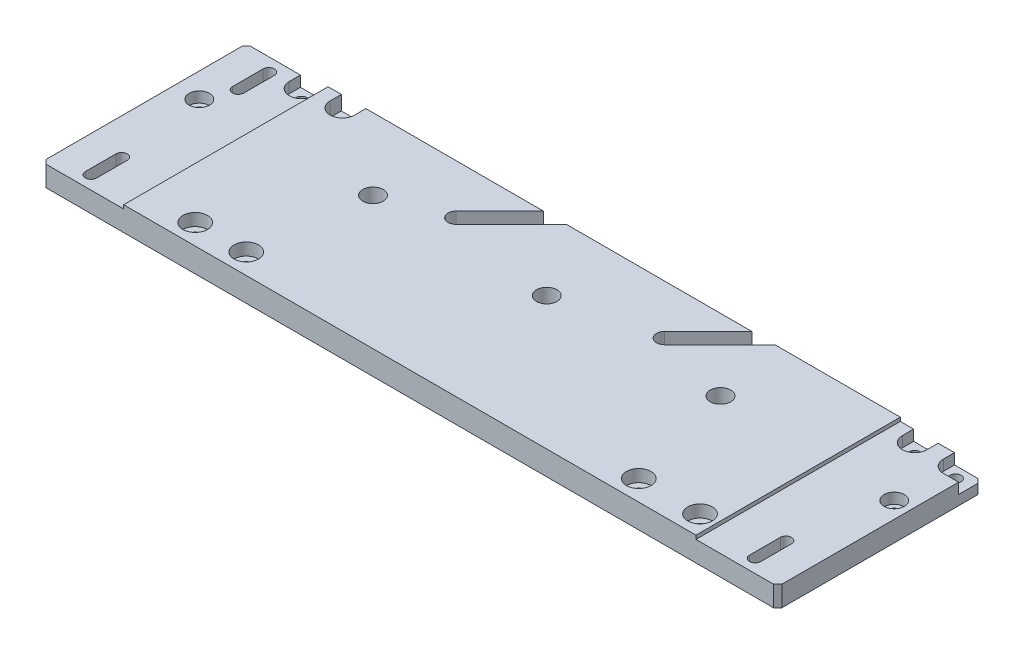
from build123d import *

# Parameters (mm, degrees)
SKETCH1_W           = 360
SKETCH1_H           = 100
BOSS_EXTRUDE1_DEPTH = 10
SKETCH2_W           = 280
SKETCH2_H           = 100
BOSS_EXTRUDE2_DEPTH = 1.8
SKETCH3_R           = 4
CUT_EXTRUDE1_DEPTH  = 188.187713272
CUT_EXTRUDE2_DEPTH  = 39
CUT_EXTRUDE3_DEPTH  = 39
CHAMFER1_SIZE       = 2
SKETCH6_R           = 2.75
CUT_EXTRUDE4_DEPTH  = 188.187713272
SKETCH7_R           = 6
CUT_EXTRUDE5_DEPTH  = 6
SKETCH8_R           = 2.75
CUT_EXTRUDE6_DEPTH  = 19
SKETCH9_R           = 6
CUT_EXTRUDE7_DEPTH  = 7
SKETCH11_W          = 12
SKETCH11_H          = 11.502298529
SKETCH11_H_2        = 11
CUT_EXTRUDE8_DEPTH  = 7
SKETCH12_R          = 2.75
CUT_EXTRUDE9_DEPTH  = 188.187713272
LPATTERN1_COUNT     = 5
LPATTERN1_PITCH     = 85
SKETCH13_R          = 5
CUT_EXTRUDE10_DEPTH = 7
SKETCH14_R          = 2.75
CUT_EXTRUDE11_DEPTH = 10
SKETCH15_R          = 6
CUT_EXTRUDE12_DEPTH = 5.2
SKETCH16_W          = 12
SKETCH16_H          = 11
CUT_EXTRUDE13_DEPTH = 5.2
SKETCH17_W          = 12
SKETCH17_H          = 12
CUT_EXTRUDE14_DEPTH = 5.2


with BuildPart() as part:
    # Sketch1 → Boss-Extrude1 (new body)
    with BuildSketch(Plane(origin=(0, 0, 0), x_dir=(1, 0, 0), z_dir=(0, 1, 0))):
        Rectangle(SKETCH1_W, SKETCH1_H)
    extrude(amount=BOSS_EXTRUDE1_DEPTH)

    # Sketch2 → Boss-Extrude2 (add)
    with BuildSketch(Plane(origin=(0, 10, 0), x_dir=(1, 0, 0), z_dir=(0, 1, 0))):
        Rectangle(SKETCH2_W, SKETCH2_H)
    extrude(amount=BOSS_EXTRUDE2_DEPTH)

    # Sketch3 → Cut-Extrude1 (cut, through all)
    with BuildSketch(Plane.XZ):
        with Locations(Location((-39, -40, 0), (0, 0, 270))):
            Circle(SKETCH3_R)
        with Locations(Location((63, -40, 0), (0, 0, 270))):
            Circle(SKETCH3_R)
    extrude(amount=-CUT_EXTRUDE1_DEPTH, mode=Mode.SUBTRACT)

    # Sketch4 → Cut-Extrude2 (cut)
    with BuildSketch(Plane.XZ):
        with BuildLine():
            Line((51.686291501, -23.029437252), (79.970562748, -51.313708499))
            ThreePointArc((79.970562748, -51.313708499), (79.970562748, -56.970562748), (74.313708499, -56.970562748))
            Line((74.313708499, -56.970562748), (46.029437252, -28.686291501))
            ThreePointArc((46.029437252, -28.686291501), (46.029437252, -23.029437252), (51.686291501, -23.029437252))
        make_face()
        with BuildLine():
            Line((-50.313708499, -23.029437252), (-22.029437252, -51.313708499))
            ThreePointArc((-22.029437252, -51.313708499), (-22.029437252, -56.970562748), (-27.686291501, -56.970562748))
            Line((-27.686291501, -56.970562748), (-55.970562748, -28.686291501))
            ThreePointArc((-55.970562748, -28.686291501), (-55.970562748, -23.029437252), (-50.313708499, -23.029437252))
        make_face()
    extrude(amount=-CUT_EXTRUDE2_DEPTH, mode=Mode.SUBTRACT)

    # Sketch5 → Cut-Extrude3 (cut)
    with BuildSketch(Plane.XZ):
        with BuildLine():
            Line((-159.753978998, 43.501457769), (-159.746021776, 28.501459879))
            ThreePointArc((-159.746021776, 28.501459879), (-162.494562565, 25.750001442), (-165.246021002, 28.498542231))
            Line((-165.246021002, 28.498542231), (-165.253978224, 43.498540121))
            ThreePointArc((-165.253978224, 43.498540121), (-162.505437435, 46.249998558), (-159.753978998, 43.501457769))
        make_face()
        with BuildLine():
            Line((159.75, 43.5), (159.75, 28.5))
            ThreePointArc((159.75, 28.5), (162.5, 25.75), (165.25, 28.5))
            Line((165.25, 28.5), (165.25, 43.5))
            ThreePointArc((165.25, 43.5), (162.5, 46.25), (159.75, 43.5))
        make_face()
        with BuildLine():
            Line((-159.753978998, -43.501457769), (-159.746021776, -28.501459879))
            ThreePointArc((-159.746021776, -28.501459879), (-162.494562565, -25.750001442), (-165.246021002, -28.498542231))
            Line((-165.246021002, -28.498542231), (-165.253978224, -43.498540121))
            ThreePointArc((-165.253978224, -43.498540121), (-162.505437435, -46.249998558), (-159.753978998, -43.501457769))
        make_face()
    extrude(amount=-CUT_EXTRUDE3_DEPTH, mode=Mode.SUBTRACT)

    # Chamfer1
    chamfer1_edges = [part.edges().sort_by_distance(p)[0] for p in [
        (180, 5, 50),
        (-180, 5, 50),
        (-180, 5, -50),
        (180, 5, -50),
    ]]
    chamfer(chamfer1_edges, length=CHAMFER1_SIZE)

    # Sketch6 → Cut-Extrude4 (cut, through all)
    with BuildSketch(Plane(origin=(0, 11.8, 0), x_dir=(1, 0, 0), z_dir=(0, 1, 0))):
        with Locations(Location((132, -40, 0), (0, 0, 270))):
            Circle(SKETCH6_R)
        with Locations(Location((102, -40, 0), (0, 0, 270))):
            Circle(SKETCH6_R)
        with Locations(Location((-90, -40, 0), (0, 0, 270))):
            Circle(SKETCH6_R)
        with Locations(Location((-115, -40, 0), (0, 0, 270))):
            Circle(SKETCH6_R)
    extrude(amount=-CUT_EXTRUDE4_DEPTH, mode=Mode.SUBTRACT)

    # Sketch7 → Cut-Extrude5 (cut)
    with BuildSketch(Plane(origin=(0, 11.8, 0), x_dir=(1, 0, 0), z_dir=(0, 1, 0))):
        with Locations(Location((-115, -40, 0), (0, 0, 270))):
            Circle(SKETCH7_R)
        with Locations(Location((-90, -40, 0), (0, 0, 270))):
            Circle(SKETCH7_R)
        with Locations(Location((102, -40, 0), (0, 0, 270))):
            Circle(SKETCH7_R)
        with Locations(Location((132, -40, 0), (0, 0, 270))):
            Circle(SKETCH7_R)
    extrude(amount=-CUT_EXTRUDE5_DEPTH, mode=Mode.SUBTRACT)

    # Sketch8 → Cut-Extrude6 (cut)
    with BuildSketch(Plane(origin=(0, 11.8, 0), x_dir=(1, 0, 0), z_dir=(0, 1, 0))):
        with Locations(Location((-147.5, 44.5, 0), (0, 0, 270))):
            Circle(SKETCH8_R)
        with Locations(Location((-127.5, 44.5, 0), (0, 0, 270))):
            Circle(SKETCH8_R)
    extrude(amount=-CUT_EXTRUDE6_DEPTH, mode=Mode.SUBTRACT)

    # Sketch9 → Cut-Extrude7 (cut)
    with BuildSketch(Plane(origin=(0, 11.8, 0), x_dir=(1, 0, 0), z_dir=(0, 1, 0))):
        with Locations((-147.5, 44.5)):
            Circle(SKETCH9_R)
        with Locations((-127.5, 44.5)):
            Circle(SKETCH9_R)
    extrude(amount=-CUT_EXTRUDE7_DEPTH, mode=Mode.SUBTRACT)

    # Sketch11 → Cut-Extrude8 (cut)
    with BuildSketch(Plane(origin=(0, 11.8, 0), x_dir=(1, 0, 0), z_dir=(0, 1, 0))):
        with Locations((-147.5, 50.251149265)):
            Rectangle(SKETCH11_W, SKETCH11_H)
        with Locations((-127.5, 50)):
            Rectangle(SKETCH11_W, SKETCH11_H_2)
    extrude(amount=-CUT_EXTRUDE8_DEPTH, mode=Mode.SUBTRACT)

    # Sketch12 → Cut-Extrude9 (cut, through all)
    with BuildSketch(Plane(origin=(0, 11.8, 0), x_dir=(1, 0, 0), z_dir=(0, 1, 0))):
        with Locations(Location((-168, 15, 0), (0, 0, 270))):
            Circle(SKETCH12_R)
    cut_extrude9 = extrude(amount=-CUT_EXTRUDE9_DEPTH, mode=Mode.SUBTRACT)

    # LPattern1: Cut-Extrude9 ×5
    with Locations(*[(i * LPATTERN1_PITCH, 0, 0) for i in range(1, LPATTERN1_COUNT)]):
        add(cut_extrude9, mode=Mode.SUBTRACT)

    # Sketch13 → Cut-Extrude10 (cut)
    with BuildSketch(Plane(origin=(0, 11.8, 0), x_dir=(1, 0, 0), z_dir=(0, 1, 0))):
        with Locations(Location((172, 15, 0), (0, 0, 270))):
            Circle(SKETCH13_R)
        with Locations(Location((87, 15, 0), (0, 0, 270))):
            Circle(SKETCH13_R)
        with Locations(Location((2, 15, 0), (0, 0, 270))):
            Circle(SKETCH13_R)
        with Locations(Location((-83, 15, 0), (0, 0, 270))):
            Circle(SKETCH13_R)
        with Locations(Location((-168, 15, 0), (0, 0, 270))):
            Circle(SKETCH13_R)
    extrude(amount=-CUT_EXTRUDE10_DEPTH, mode=Mode.SUBTRACT)

    # Sketch14 → Cut-Extrude11 (cut)
    with BuildSketch(Plane.XZ):
        with Locations(Location((152.5, -44.5, 0), (0, 0, 270))):
            Circle(SKETCH14_R)
        with Locations(Location((172.5, -44.5, 0), (0, 0, 270))):
            Circle(SKETCH14_R)
    extrude(amount=-CUT_EXTRUDE11_DEPTH, mode=Mode.SUBTRACT)

    # Sketch15 → Cut-Extrude12 (cut)
    with BuildSketch(Plane(origin=(0, 10, 0), x_dir=(1, 0, 0), z_dir=(0, 1, 0))):
        with Locations((152.5, 44.5)):
            Circle(SKETCH15_R)
        with Locations((172.5, 44.5)):
            Circle(SKETCH15_R)
    extrude(amount=-CUT_EXTRUDE12_DEPTH, mode=Mode.SUBTRACT)

    # Sketch16 → Cut-Extrude13 (cut)
    with BuildSketch(Plane(origin=(0, 10, 0), x_dir=(1, 0, 0), z_dir=(0, 1, 0))):
        with Locations((152.5, 50)):
            Rectangle(SKETCH16_W, SKETCH16_H)
        with Locations((172.5, 50)):
            Rectangle(SKETCH16_W, SKETCH16_H)
    extrude(amount=-CUT_EXTRUDE13_DEPTH, mode=Mode.SUBTRACT)

    # Sketch17 → Cut-Extrude14 (cut)
    with BuildSketch(Plane(origin=(0, 10, 0), x_dir=(1, 0, 0), z_dir=(0, 1, 0))):
        with Locations((178.5, 44.5)):
            Rectangle(SKETCH17_W, SKETCH17_H)
    extrude(amount=-CUT_EXTRUDE14_DEPTH, mode=Mode.SUBTRACT)


solid = part.part
